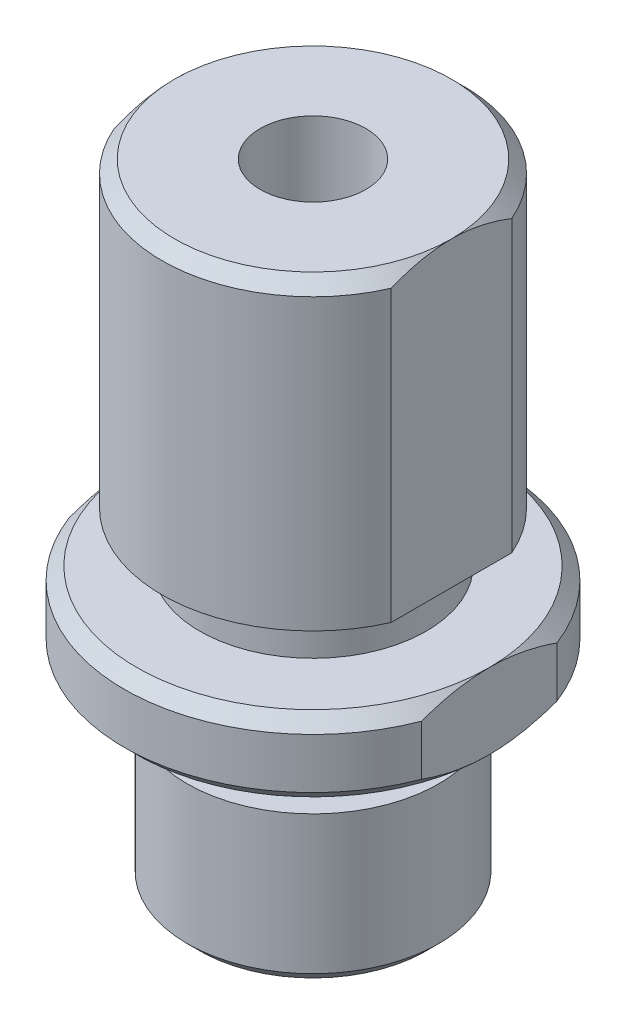
from build123d import *
from build123d.topology import SkipClean

# Parameters (mm, degrees)
SKETCH_1_R          = 6
EXTRUDE_1_DEPTH     = 14
SKETCH_2_R          = 7.5
EXTRUDE_2_DEPTH     = 3
SKETCH_3_R          = 5
EXTRUDE_3_DEPTH     = 8
SKETCH_8_R          = 2.1
CUT_EXTRUDE_1_DEPTH = 28.156951228
CHAMFER_1_SIZE      = 0.5
SKETCH_9_W          = 14.77232069
SKETCH_9_H          = 13.551998546
CUT_EXTRUDE_2_DEPTH = 4.5
CHAMFER_2_SIZE      = 0.5
SKETCH_11_W         = 9.643873146
SKETCH_11_H         = 27.541523797
SKETCH_11_W_2       = 13.856983611
CUT_EXTRUDE_3_DEPTH = 10
SKETCH_12_W         = 9.292809808
SKETCH_12_H         = 2
SKETCH_13_W         = 6.810956272
SKETCH_13_H         = 2


with BuildPart() as part:
    # 草图1 → 凸台-拉伸1 (new body)
    with BuildSketch(Plane(origin=(0, 0, 0), x_dir=(1, 0, 0), z_dir=(0, 1, 0))):
        with Locations(Location((0, 0, 0), (0, 0, 270))):
            Circle(SKETCH_1_R)
    extrude(amount=-EXTRUDE_1_DEPTH)

    # 草图2 → 凸台-拉伸2 (add)
    with BuildSketch(Plane.XZ.offset(14)):
        with Locations(Location((0, 0, 0), (0, 0, 270))):
            Circle(SKETCH_2_R)
    extrude(amount=EXTRUDE_2_DEPTH)

    # 草图3 → 凸台-拉伸3 (add)
    with BuildSketch(Plane.XZ.offset(17)):
        with Locations(Location((0, 0, 0), (0, 0, 270))):
            Circle(SKETCH_3_R)
    extrude(amount=EXTRUDE_3_DEPTH)

    # 草图8 → 切除-拉伸1 (cut, through all)
    with BuildSketch(Plane.XZ):
        with Locations(Location((0, 0, 0), (0, 0, 270))):
            Circle(SKETCH_8_R)
    extrude(amount=CUT_EXTRUDE_1_DEPTH, mode=Mode.SUBTRACT)

    # 倒角1
    chamfer_1_edges = [part.edges().sort_by_distance(p)[0] for p in [
        (0, 0, -6),
        (0, -14, 7.5),
        (0, -17, 7.5),
    ]]
    chamfer(chamfer_1_edges, length=CHAMFER_1_SIZE)

    # 草图9 → 切除-拉伸2 (cut, symmetric)
    with SkipClean():  # the faces are left unmerged after this step: merging them gives an invalid solid
        with BuildSketch(Plane.XY):
            with Locations((14.386160345, -10.910714622)):
                Rectangle(SKETCH_9_W, SKETCH_9_H)
        cut_extrude_2 = extrude(amount=CUT_EXTRUDE_2_DEPTH, both=True, mode=Mode.SUBTRACT)

    # 镜向1: 切除-拉伸2 across plane
    add(cut_extrude_2.mirror(Plane(origin=(0, 0, 0), x_dir=(0, 0, 1), z_dir=(1, 0, 0))), mode=Mode.SUBTRACT)

    # 倒角2
    chamfer_2_edges = [part.edges().sort_by_distance(p)[0] for p in [
        (0, -25, 5),
    ]]
    chamfer(chamfer_2_edges, length=CHAMFER_2_SIZE)

    # 草图11 → 切除-拉伸3 (cut, symmetric)
    with BuildSketch(Plane.XY):
        with Locations((10.321936573, -0.229238102)):
            Rectangle(SKETCH_11_W, SKETCH_11_H)
        with Locations((-12.428491806, -0.229238102)):
            Rectangle(SKETCH_11_W_2, SKETCH_11_H)
    extrude(amount=CUT_EXTRUDE_3_DEPTH, both=True, mode=Mode.SUBTRACT)

    # 草图12 → 切除-旋转2 (revolve, cut)
    with BuildSketch(Plane.XY, mode=Mode.PRIVATE) as cut_revolve_2_sk:
        with Locations((-8.646404904, -18)):
            Rectangle(SKETCH_12_W, SKETCH_12_H)
    revolve(cut_revolve_2_sk.sketch.rotate(Axis((0, -17, 0), (0, 1, 0)), 90), axis=Axis((0, -17, 0), (0, 1, 0)), mode=Mode.SUBTRACT)

    # 草图13 → 切除-旋转3 (revolve, cut)
    with BuildSketch(Plane.XY, mode=Mode.PRIVATE) as cut_revolve_3_sk:
        with Locations((-7.905478136, -13)):
            Rectangle(SKETCH_13_W, SKETCH_13_H)
    revolve(cut_revolve_3_sk.sketch.rotate(Axis((0, -14, 0), (0, 1, 0)), 270), axis=Axis((0, -14, 0), (0, 1, 0)), mode=Mode.SUBTRACT)


solid = part.part
